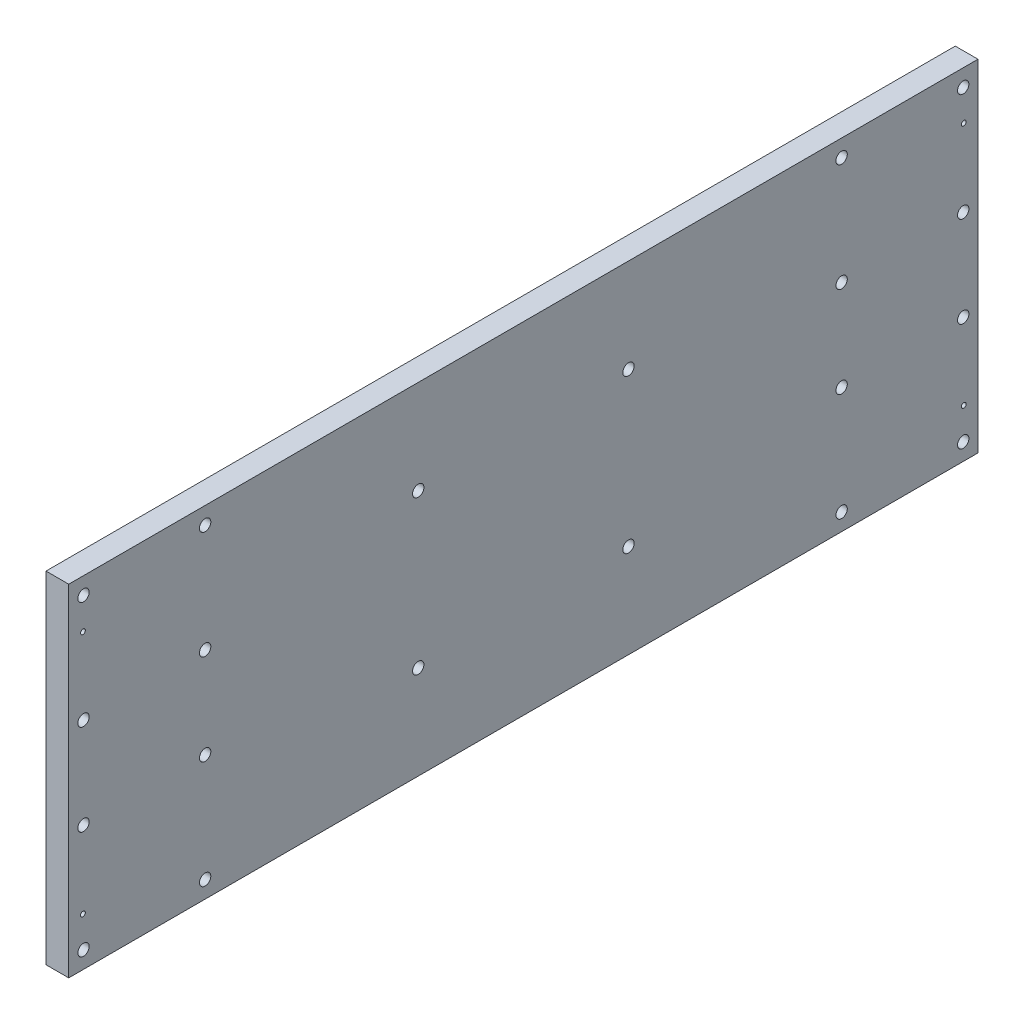
SolidWorks part; units mm, degrees
ref_plane "Front Plane" through (0, 0, 0) normal (0, 0, 1) x (1, 0, 0)
ref_plane "Top Plane" through (0, 0, 0) normal (0, 1, 0) x (1, 0, 0)
ref_plane "Right Plane" through (0, 0, 0) normal (1, 0, 0) x (0, 0, -1)
sketch "Sketch1" plane through (0, 0, 0) normal (1, 0, 0) x (0, 0, -1)
  line L1 (-400, -150) -> (400, -150)
  line L2 (-400, -150) -> (-400, 150)
  line L3 (-400, 150) -> (400, 150)
  line L4 (400, -150) -> (400, 150)
  line L5 (-400, -150) -> (400, 150) construction
  line L6 (-400, 150) -> (400, -150) construction
  point P0 (0, 0)
  dimension "D1" = 800
  dimension "D2" = 300
extrude "Boss-Extrude1" add sketch "Sketch1" along normal blind 20
sketch "Sketch2" plane through (20, 0, 0) normal (1, 0, 0) x (0, 0, -1)
  line L0 (-400, 150) -> (-400, -150) construction
  line L1 (400, 150) -> (-400, 150) construction
  line L2 (0, 150) -> (0, -150) construction
  line L3 (-400, -150) -> (400, -150) construction
  line L4 (-400, 0) -> (400, 0) construction
  line L5 (400, -150) -> (400, 150) construction
  circle A0 centre (-387, 135) radius 5
  circle A1 centre (-280, 135) radius 5
  circle A2 centre (-280, 40) radius 5
  circle A3 centre (-387, 40) radius 5
  circle A4 centre (-280, -40) radius 5
  circle A5 centre (-280, -135) radius 5
  circle A6 centre (-387, -135) radius 5
  circle A7 centre (-387, -40) radius 5
  circle A8 centre (280, -40) radius 5
  circle A9 centre (280, -135) radius 5
  circle A10 centre (387, -135) radius 5
  circle A11 centre (387, -40) radius 5
  circle A12 centre (280, 135) radius 5
  circle A13 centre (387, 135) radius 5
  circle A14 centre (387, 40) radius 5
  circle A15 centre (280, 40) radius 5
  dimension "D1" = 10
  dimension "D2" = 13
  dimension "D3" = 15
  dimension "D6" = 107
  dimension "D7" = 95
  dimension "D8" = 13
  dimension "D4" = 2
  dimension "D5" = 2
extrude "Cut-Extrude1" cut sketch "Sketch2" against normal blind 20
sketch "Sketch3" plane through (20, 0, 0) normal (1, 0, 0) x (0, 0, -1)
  line L0 (400, -150) -> (400, 150) construction
  line L1 (-400, -150) -> (400, -150) construction
  line L2 (-183.0407, 0) -> (141.0995, 0) construction
  line L3 (0, 110.4821) -> (0, -73.25) construction
  circle A0 centre (387.5, -107.5) radius 2.1
  circle A1 centre (387.5, 107.5) radius 2.1
  circle A2 centre (-387.5, -107.5) radius 2.1
  circle A3 centre (-387.5, 107.5) radius 2.1
  dimension "D1" = 4.2
  dimension "D2" = 12.5
  dimension "D3" = 42.5
extrude "Cut-Extrude2" cut sketch "Sketch3" against normal blind 65
sketch "Sketch4" plane through (20, 0, 0) normal (1, 0, 0) x (0, 0, -1)
  line L0 (-400, 0) -> (400, 0) construction
  line L1 (-400, 150) -> (-400, -150) construction
  line L2 (400, -150) -> (400, 150) construction
  line L3 (0, 150) -> (0, -150) construction
  line L4 (400, 150) -> (-400, 150) construction
  line L5 (-400, -150) -> (400, -150) construction
  circle A0 centre (-92.5, 67.5) radius 5
  circle A1 centre (92.5, 67.5) radius 5
  circle A2 centre (92.5, -67.5) radius 5
  circle A3 centre (-92.5, -67.5) radius 5
  dimension "D3" = 10
  dimension "D1" = 92.5
  dimension "D2" = 67.5
extrude "Cut-Extrude3" cut sketch "Sketch4" against normal blind 226
